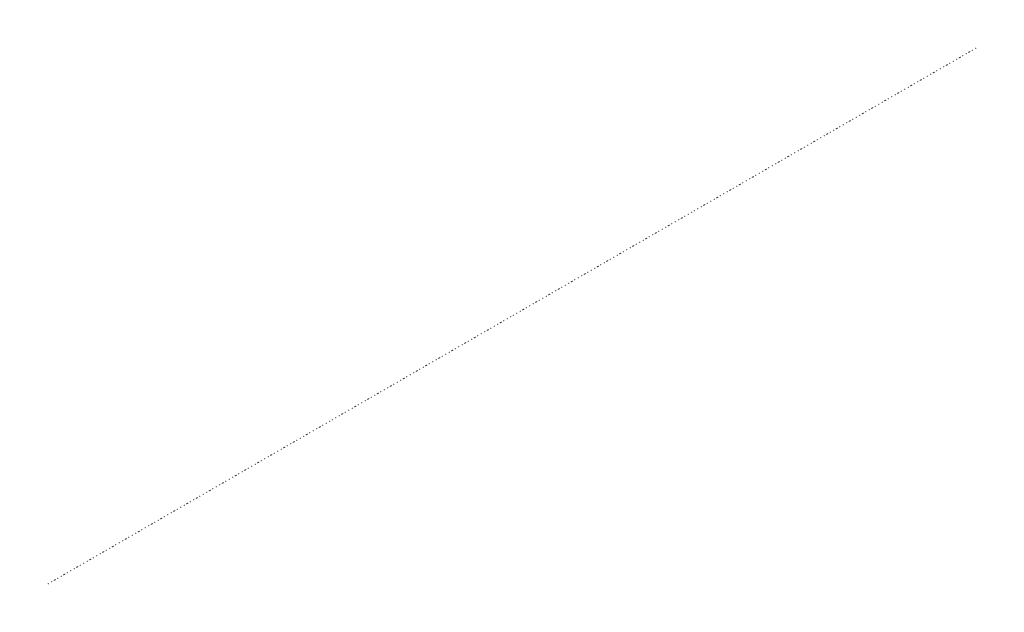
from build123d import *

# Parameters (mm, degrees)
SKETCH1_R           = 0.0625
BOSS_EXTRUDE1_DEPTH = 1900


with BuildPart() as part:
    # Sketch1 → Boss-Extrude1 (new body)
    with BuildSketch(Plane.XY):
        Circle(SKETCH1_R)
    extrude(amount=BOSS_EXTRUDE1_DEPTH)


solid = part.part
